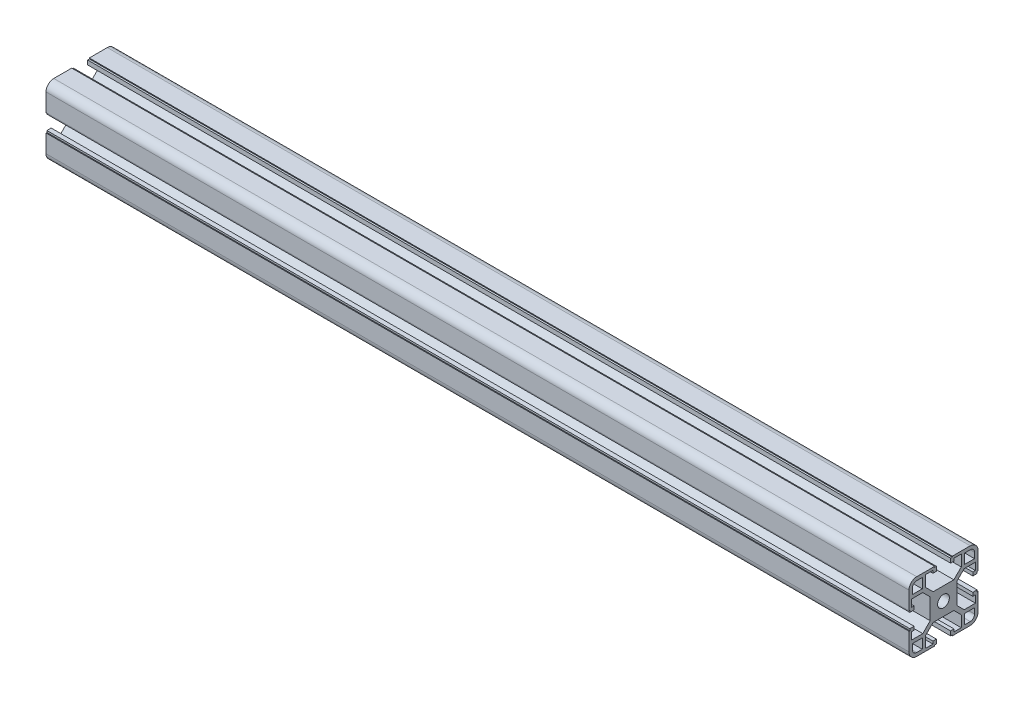
from build123d import *

# Parameters (mm, degrees)
SKETCH1_R                                = 3.4
ALUMINUM_PROFILE_40_X_40B_X_R4_5_1_DEPTH = 500


with BuildPart() as part:
    # Sketch1 → Aluminum profile 40 X 40B X R4.5(1) (new body)
    with BuildSketch(Plane.YZ):
        with BuildLine():
            Line((-5.1, 20), (-5.1, 19.5))
            Line((-5.1, 19.5), (-4.1, 19.5))
            Line((-4.1, 19.5), (-4.1, 17))
            Line((-4.1, 17), (-6.1, 17))
            Line((-6.1, 17), (-6.1, 18.5))
            Line((-6.1, 18.5), (-10.3, 18.5))
            Line((-10.3, 18.5), (-10.3, 12))
            Line((-10.3, 12), (-6, 7.7))
            Line((-6, 7.7), (6, 7.7))
            Line((6, 7.7), (10.3, 12))
            Line((10.3, 12), (10.3, 18.5))
            Line((10.3, 18.5), (6.1, 18.5))
            Line((6.1, 18.5), (6.1, 17))
            Line((6.1, 17), (4.1, 17))
            Line((4.1, 17), (4.1, 19.5))
            Line((4.1, 19.5), (5.1, 19.5))
            Line((5.1, 19.5), (5.1, 20))
            Line((5.1, 20), (15.5, 20))
            ThreePointArc((15.5, 20), (18.681980515, 18.681980515), (20, 15.5))
            Line((20, 15.5), (20, 5.1))
            Line((20, 5.1), (19.5, 5.1))
            Line((19.5, 5.1), (19.5, 4.1))
            Line((19.5, 4.1), (17, 4.1))
            Line((17, 4.1), (17, 6.1))
            Line((17, 6.1), (18.5, 6.1))
            Line((18.5, 6.1), (18.5, 10.3))
            Line((18.5, 10.3), (12, 10.3))
            Line((12, 10.3), (7.7, 6))
            Line((7.7, 6), (7.7, -6))
            Line((7.7, -6), (12, -10.3))
            Line((12, -10.3), (18.5, -10.3))
            Line((18.5, -10.3), (18.5, -6.1))
            Line((18.5, -6.1), (17, -6.1))
            Line((17, -6.1), (17, -4.1))
            Line((17, -4.1), (19.5, -4.1))
            Line((19.5, -4.1), (19.5, -5.1))
            Line((19.5, -5.1), (20, -5.1))
            Line((20, -5.1), (20, -15.5))
            ThreePointArc((20, -15.5), (18.681980515, -18.681980515), (15.5, -20))
            Line((15.5, -20), (5.1, -20))
            Line((5.1, -20), (5.1, -19.5))
            Line((5.1, -19.5), (4.1, -19.5))
            Line((4.1, -19.5), (4.1, -17))
            Line((4.1, -17), (6.1, -17))
            Line((6.1, -17), (6.1, -18.5))
            Line((6.1, -18.5), (10.3, -18.5))
            Line((10.3, -18.5), (10.3, -12))
            Line((10.3, -12), (6, -7.7))
            Line((6, -7.7), (-6, -7.7))
            Line((-6, -7.7), (-10.3, -12))
            Line((-10.3, -12), (-10.3, -18.5))
            Line((-10.3, -18.5), (-6.1, -18.5))
            Line((-6.1, -18.5), (-6.1, -17))
            Line((-6.1, -17), (-4.1, -17))
            Line((-4.1, -17), (-4.1, -19.5))
            Line((-4.1, -19.5), (-5.1, -19.5))
            Line((-5.1, -19.5), (-5.1, -20))
            Line((-5.1, -20), (-15.5, -20))
            ThreePointArc((-15.5, -20), (-18.681980515, -18.681980515), (-20, -15.5))
            Line((-20, -15.5), (-20, -5.1))
            Line((-20, -5.1), (-19.5, -5.1))
            Line((-19.5, -5.1), (-19.5, -4.1))
            Line((-19.5, -4.1), (-17, -4.1))
            Line((-17, -4.1), (-17, -6.1))
            Line((-17, -6.1), (-18.5, -6.1))
            Line((-18.5, -6.1), (-18.5, -10.3))
            Line((-18.5, -10.3), (-12, -10.3))
            Line((-12, -10.3), (-7.7, -6))
            Line((-7.7, -6), (-7.7, 6))
            Line((-7.7, 6), (-12, 10.3))
            Line((-12, 10.3), (-18.5, 10.3))
            Line((-18.5, 10.3), (-18.5, 6.1))
            Line((-18.5, 6.1), (-17, 6.1))
            Line((-17, 6.1), (-17, 4.1))
            Line((-17, 4.1), (-19.5, 4.1))
            Line((-19.5, 4.1), (-19.5, 5.1))
            Line((-19.5, 5.1), (-20, 5.1))
            Line((-20, 5.1), (-20, 15.5))
            ThreePointArc((-20, 15.5), (-18.681980515, 18.681980515), (-15.5, 20))
            Line((-15.5, 20), (-5.1, 20))
        make_face()
        Circle(SKETCH1_R, mode=Mode.SUBTRACT)
        with BuildLine():
            Line((12.3, 18), (15.5, 18))
            ThreePointArc((15.5, 18), (17.267766953, 17.267766953), (18, 15.5))
            Line((18, 15.5), (18, 12.3))
            Line((18, 12.3), (12.3, 12.3))
            Line((12.3, 12.3), (12.3, 18))
        make_face(mode=Mode.SUBTRACT)
        with BuildLine():
            Line((-15.5, 18), (-12.3, 18))
            Line((-12.3, 18), (-12.3, 12.3))
            Line((-12.3, 12.3), (-18, 12.3))
            Line((-18, 12.3), (-18, 15.5))
            ThreePointArc((-18, 15.5), (-17.267766953, 17.267766953), (-15.5, 18))
        make_face(mode=Mode.SUBTRACT)
        with BuildLine():
            Line((-18, -12.3), (-12.3, -12.3))
            Line((-12.3, -12.3), (-12.3, -18))
            Line((-12.3, -18), (-15.5, -18))
            ThreePointArc((-15.5, -18), (-17.267766953, -17.267766953), (-18, -15.5))
            Line((-18, -15.5), (-18, -12.3))
        make_face(mode=Mode.SUBTRACT)
        with BuildLine():
            Line((12.3, -12.3), (18, -12.3))
            Line((18, -12.3), (18, -15.5))
            ThreePointArc((18, -15.5), (17.267766953, -17.267766953), (15.5, -18))
            Line((15.5, -18), (12.3, -18))
            Line((12.3, -18), (12.3, -12.3))
        make_face(mode=Mode.SUBTRACT)
    extrude(amount=ALUMINUM_PROFILE_40_X_40B_X_R4_5_1_DEPTH)


solid = part.part
